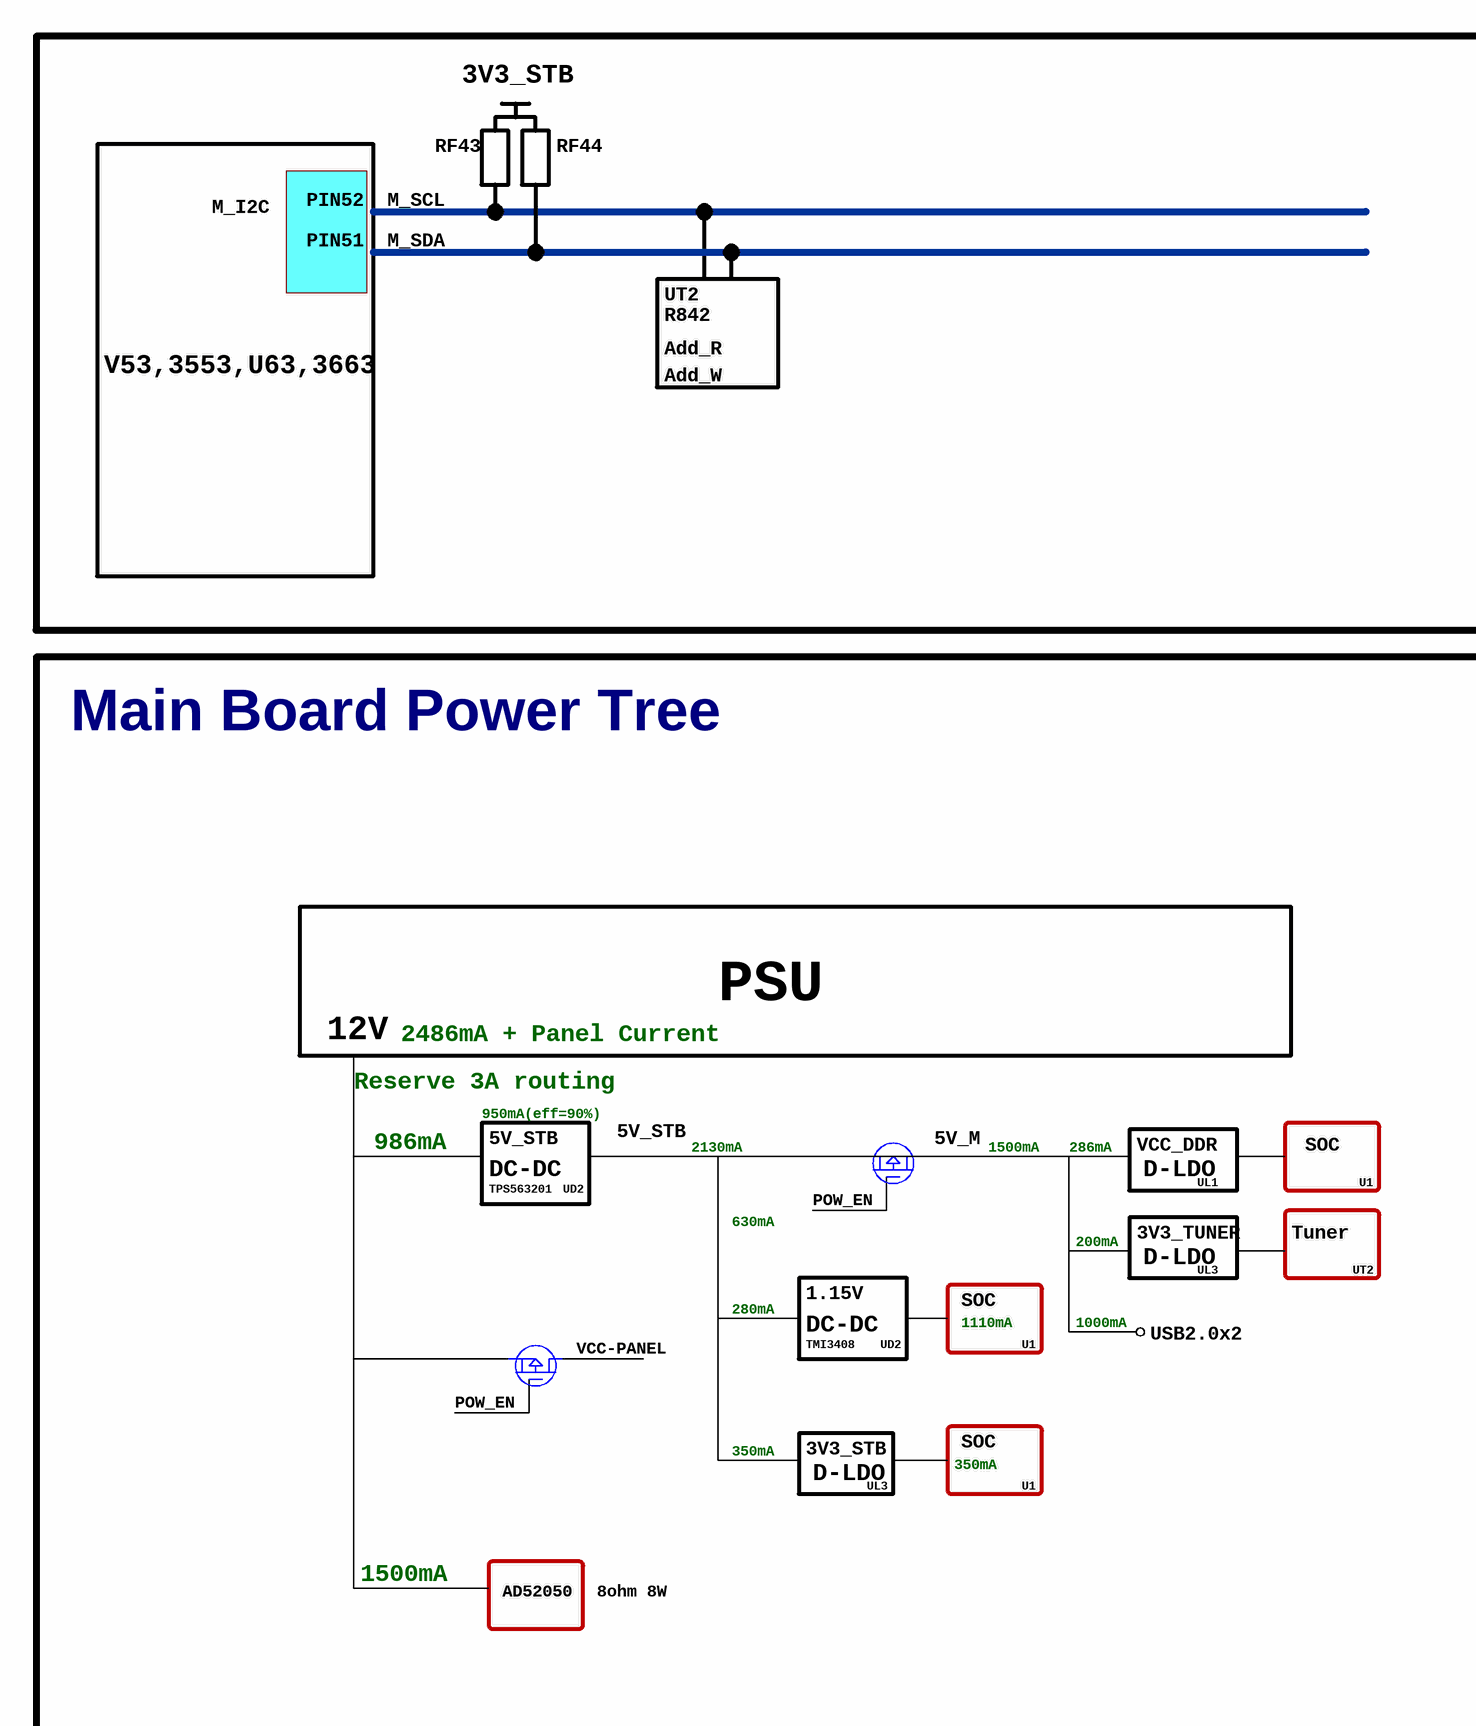
[diagram p0: MISC86372-17.SchDoc, left]
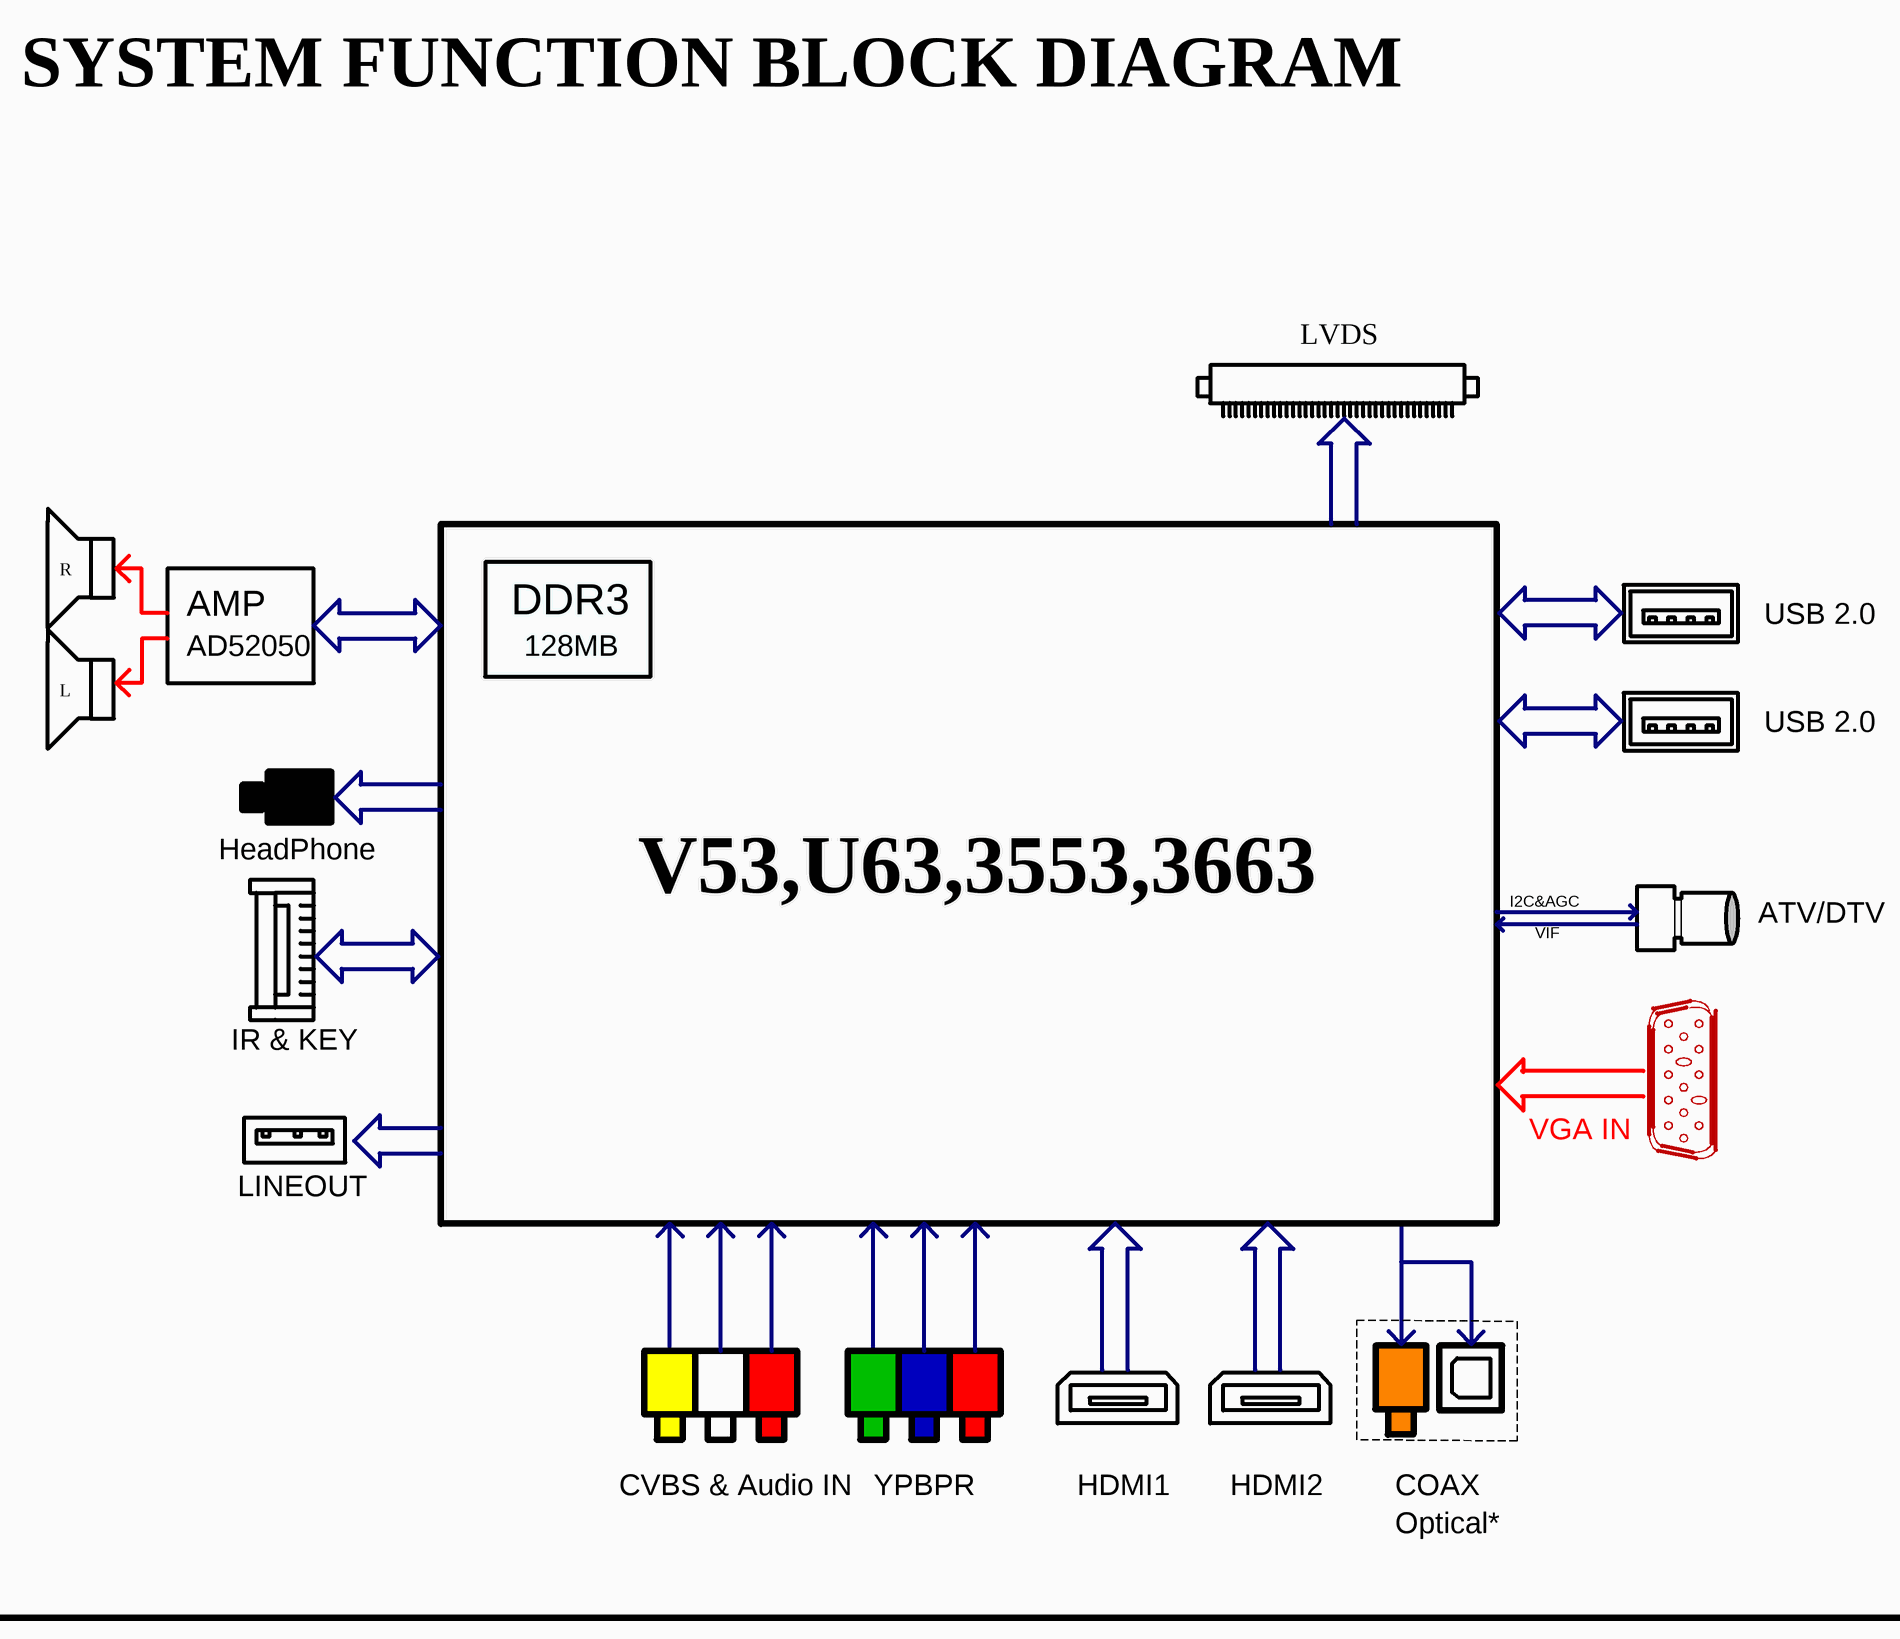
[diagram p1: MISC86372-17.SchDoc, right]
# Altium project MISC86372-32.PrjPCB (part 2 of 8)

## Sheet MISC86372-17.SchDoc
size 736 x 347 mm

### Notes on the sheet
- 3V3_STB
- RF43
- RF44
- SYSTEM FUNCTION BLOCK DIAGRAM
- M_I2C
- PIN52
- M_SCL
- PIN51
- M_SDA
- UT2
- V53,3553,U63,3663
- R842
- Add_R
- Add_W
- LVDS
- R
- Main Board Power Tree
- AMP
- AD52050
- DDR3
- 128MB
- USB 2.0
- L
- HeadPhone
- 12V
- 2486mA + Panel Current
- PSU
- V53,U63,3553,3663
- I2C&AGC
- ATV/DTV
- Reserve 3A routing
- VIF
- 986mA
- 950mA(eff=90%)
- DC-DC
- 5V_STB
- 2130mA
- 5V_M
- 1500mA
- 286mA
- VCC_DDR
- D-LDO
- UL1
- SOC
- U1
- IR & KEY
- TPS563201
- UD2
- 630mA
- POW_EN
- 200mA
- 3V3_TUNER
- Tuner
- 280mA
- 1.15V
- UL3
- VGA IN
- VCC-PANEL
- TMI3408
- 1110mA
- 1000mA
- USB2.0x2
- LINEOUT
- 350mA
- 8ohm 8W
- CVBS & Audio IN
- YPBPR
- HDMI1
- HDMI2
- COAX
- Optical*

## Sheet MISC86372-8.SchDoc
size 393 x 241 mm
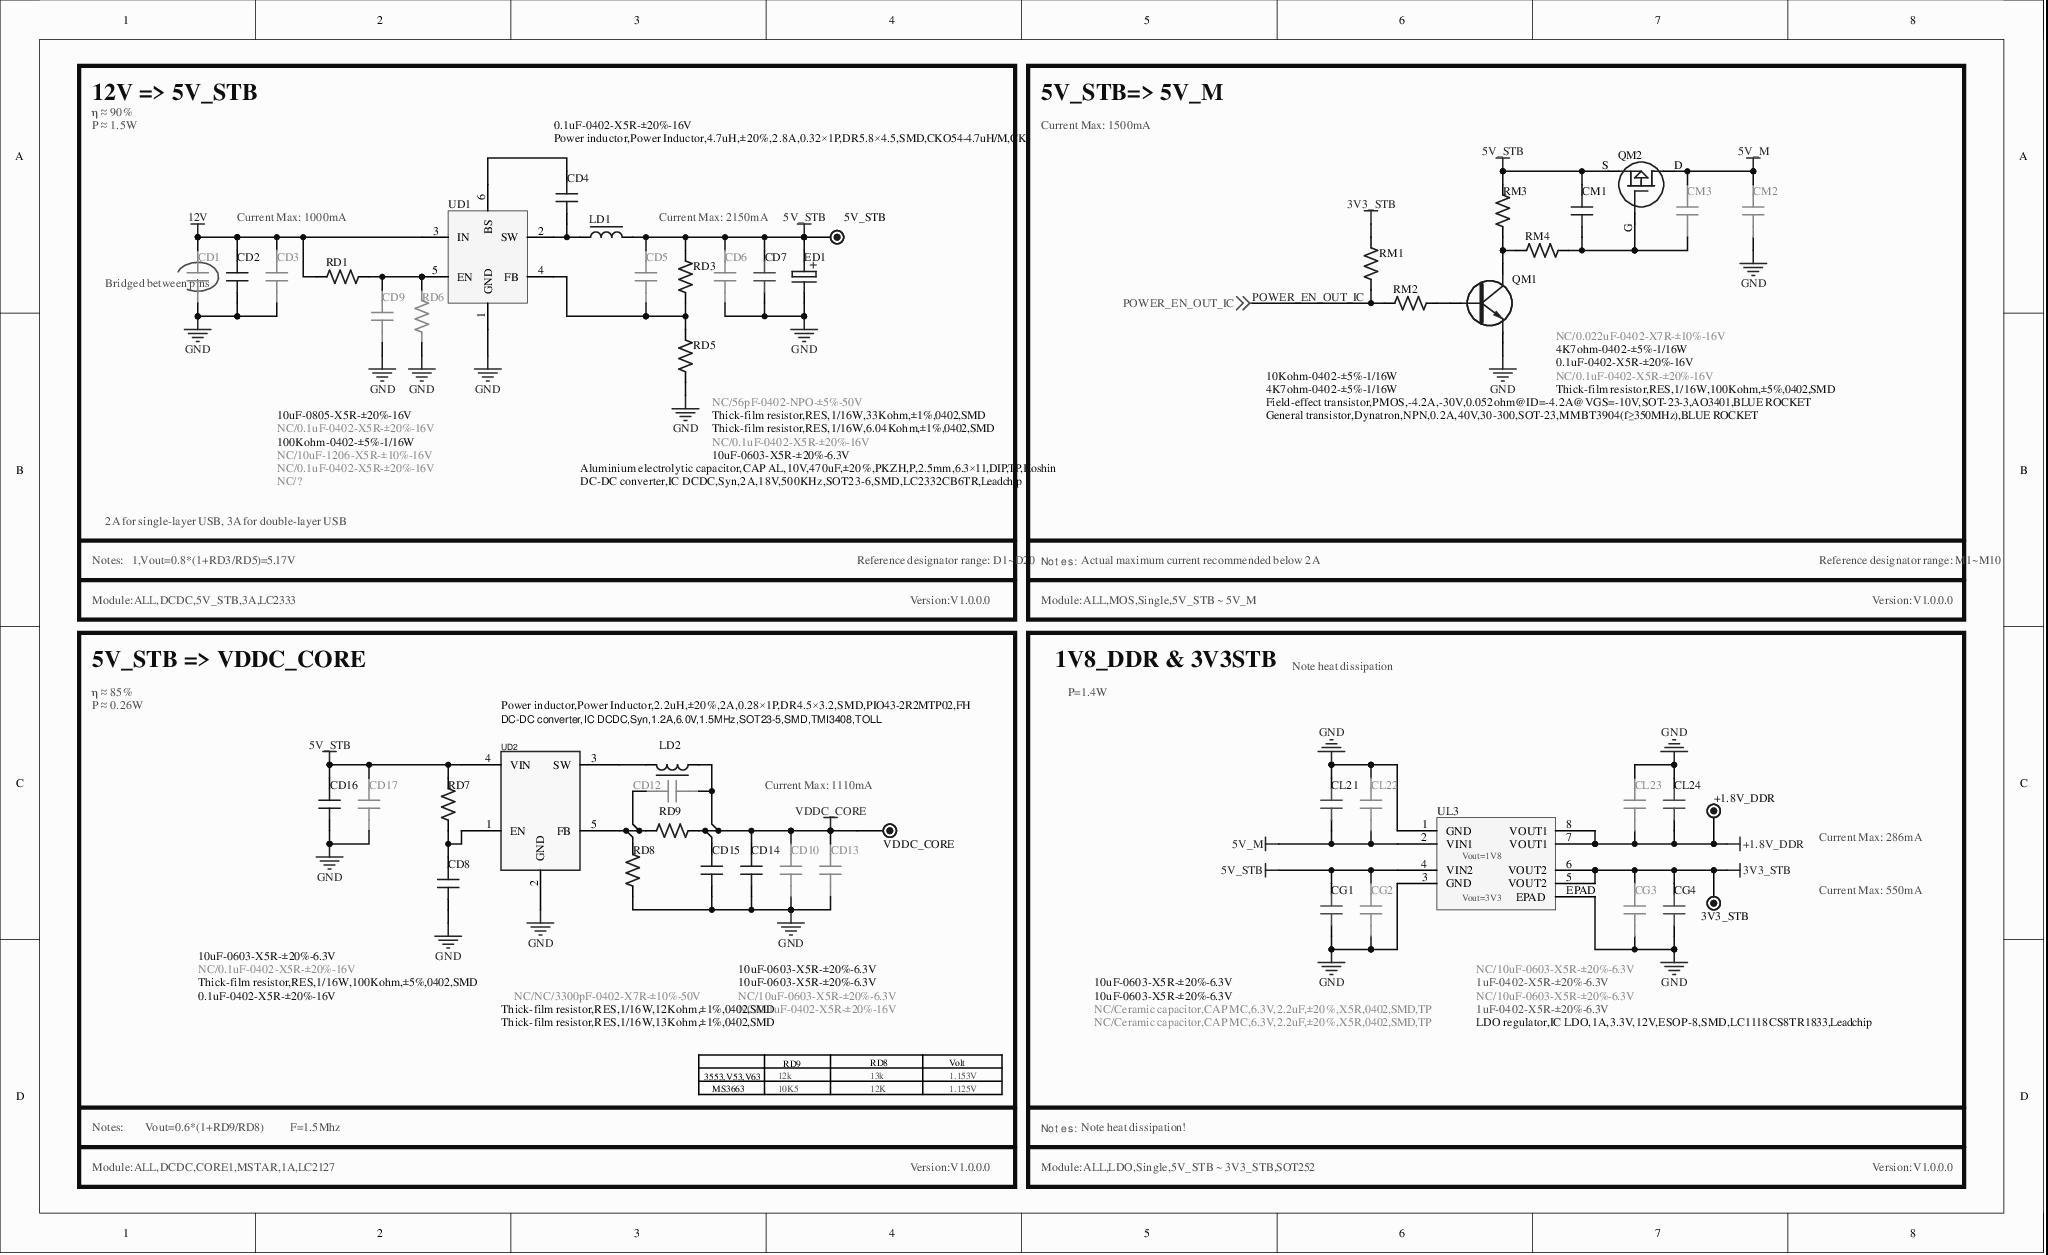
[diagram p2: MISC86372-8.SchDoc]

### Parts
3V3_STB  TEST  [TP]  (value not drawn)
5V_STB  TEST  [TP]  (value not drawn)
+1.8V_DDR  TEST  [TP]  (value not drawn)
CD1  NC/10uF-1206-X5R-±10%-16V  [C1206]
CD2  10uF-0805-X5R-±20%-16V  [C0805]
CD3  NC/0.1uF-0402-X5R-±20%-16V  [C0402]
CD4  0.1uF-0402-X5R-±20%-16V  [C0402]
CD5  NC/56pF-0402-NPO-±5%-50V  [C0402]
CD6  NC/0.1uF-0402-X5R-±20%-16V  [C0402]
CD7  10uF-0603-X5R-±20%-6.3V  [C0603]
CD8  0.1uF-0402-X5R-±20%-16V  [C0402]
CD9  NC/0.1uF-0402-X5R-±20%-16V  [C0402]
CD10  NC/10uF-0603-X5R-±20%-6.3V  [C0603]
CD12  NC/NC/3300pF-0402-X7R-±10%-50V  [C0402]
CD13  NC/0.1uF-0402-X5R-±20%-16V  [C0402]
CD14  10uF-0603-X5R-±20%-6.3V  [C0603]
CD15  10uF-0603-X5R-±20%-6.3V  [C0603]
CD16  10uF-0603-X5R-±20%-6.3V  [C0603]
CD17  NC/0.1uF-0402-X5R-±20%-16V  [C0402]
CG1  10uF-0603-X5R-±20%-6.3V  [C0603]
CG2  NC/Ceramic capacitor,CAP MC,6.3V,2.2uF,±20%,X5R,0402,SMD,TP  [C0402]
CG3  NC/10uF-0603-X5R-±20%-6.3V  [C0603]
CG4  1uF-0402-X5R-±20%-6.3V  [C0402]
CL21  10uF-0603-X5R-±20%-6.3V  [C0603]
CL22  NC/Ceramic capacitor,CAP MC,6.3V,2.2uF,±20%,X5R,0402,SMD,TP  [C0402]
CL23  NC/10uF-0603-X5R-±20%-6.3V  [C0603]
CL24  1uF-0402-X5R-±20%-6.3V  [C0402]
CM1  0.1uF-0402-X5R-±20%-16V  [C0402]
CM2  NC/0.1uF-0402-X5R-±20%-16V  [C0402]
CM3  NC/0.022uF-0402-X7R-±10%-16V  [C0402]
ED1  Aluminium electrolytic capacitor,CAP AL,10V,470uF,±20%,PKZH,P,2.5mm,6.3×11,DIP,TP,Koshin  [EC(6.3*11)-V-2.5]
LD1  Power inductor,Power Inductor,4.7uH,±20%,2.8A,0.32×1P,DR5.8×4.5,SMD,CKO54-4.7uH/M,CK  [L(5.8*4.5)-S]
LD2  Power inductor,Power Inductor,2.2uH,±20%,2A,0.28×1P,DR4.5×3.2,SMD,PIO43-2R2MTP02,FH  [L(4.5*3.5)-S]
QM1  General transistor,Dynatron,NPN,0.2A,40V,30-300,SOT-23,MMBT3904(f≥350MHz),BLUE ROCKET  [SOT-23]
QM2  Field-effect transistor,PMOS,-4.2A,-30V,0.052ohm@ID=-4.2A@VGS=-10V,SOT-23-3,AO3401,BLUE ROCKET  [SOT-23-1]
RD1  100Kohm-0402-±5%-1/16W  [R0402]
RD3  Thick-film resistor,RES,1/16W,33Kohm,±1%,0402,SMD  [R0402]
RD5  Thick-film resistor,RES,1/16W,6.04Kohm,±1%,0402,SMD  [R0402]
RD6  NC/?  [R0402]
RD7  Thick-film resistor,RES,1/16W,100Kohm,±5%,0402,SMD  [R0402]
RD8  Thick-film resistor,RES,1/16W,13Kohm,±1%,0402,SMD  [R0402]
RD9  Thick-film resistor,RES,1/16W,12Kohm,±1%,0402,SMD  [R0402]
RM1  10Kohm-0402-±5%-1/16W  [R0402]
RM2  4K7ohm-0402-±5%-1/16W  [R0402]
RM3  4K7ohm-0402-±5%-1/16W  [R0402]
RM4  Thick-film resistor,RES,1/16W,100Kohm,±5%,0402,SMD  [R0402]
UD1  DC-DC converter,IC DCDC,Syn,2A,18V,500KHz,SOT23-6,SMD,LC2332CB6TR,Leadchip  [SOT-23-6]
UD2  DC-DC converter,IC DCDC,Syn,1.2A,6.0V,1.5MHz,SOT23-5,SMD,TMI3408,TOLL  [SOT-23-5]
UL3  LDO regulator,IC LDO,1A,3.3V,12V,ESOP-8,SMD,LC1118CS8TR1833,Leadchip  [SOP8/1.27-3]
VDDC_CORE  TEST  [TP]  (value not drawn)

### Blocks framed on the sheet
12V => 5V_STB: 5V_STB CD1-CD7 CD9 ED1 LD1 RD1 RD3 RD5 RD6 UD1
5V_STB=> 5V_M: CM1-CM3 QM1 QM2 RM1-RM4
5V_STB => VDDC_CORE: CD8 CD10 CD12-CD17 LD2 RD7-RD9 UD2 VDDC_CORE
1V8_DDR & 3V3STB: 3V3_STB +1.8V_DDR CG1-CG4 CL21-CL24 UL3

### Nets
3V3_STB: 3V3_STB.1 CG3.2 CG4.1 RM1.2 UL3.5(VOUT2) UL3.6(VOUT2)
5V_M: CL21.1 CL22.1 CM2.2 CM3.1 QM2.D UL3.2(VIN1)
5V_STB: 5V_STB.1 CD5.2 CD6.2 CD7.2 CD16.2 CD17.2 CG1.2 CG2.2 CM1.2 ED1.1 LD1.2 QM2.S RD3.2 RD7.2 RM3.2 UD2.4(VIN) UL3.4(VIN2)
12V: CD1.2 CD2.1 CD3.2 RD1.1 UD1.3(IN)
+1.8V_DDR: +1.8V_DDR.1 CL23.1 CL24.2 UL3.7(VOUT1) UL3.8(VOUT1)
GND: CD1.1 CD2.2 CD3.1 CD6.1 CD7.1 CD8.1 CD9.1 CD10.1 CD13.1 CD14.1 CD15.1 CD16.1 CD17.1 CG1.1 CG2.1 CG3.1 CG4.2 CL21.2 CL22.2 CL23.2 CL24.1 CM2.1 ED1.2 QM1.E RD5.1 RD6.1 RD8.2 UD1.1(GND) UD2.2(GND) UL3.1(GND) UL3.3(GND) UL3.EPAD
VDDC_CORE: CD10.2 CD12.2 CD13.2 CD14.2 CD15.2 LD2.1 RD9.1 VDDC_CORE.1
POWER_EN_OUT_IC: RM1.1 RM2.1 ; off-sheet POWER_EN_OUT_IC
NetCD4_1: CD4.1 LD1.1 UD1.2(SW)
NetCD4_2: CD4.2 UD1.6(BS)
NetCD5_1: CD5.1 RD3.1 RD5.2 UD1.4(FB)
NetCD8_2: CD8.2 RD7.1 UD2.1(EN)
NetCD9_2: CD9.2 RD1.2 RD6.2 UD1.5(EN)
NetCD12_1: CD12.1 RD8.1 RD9.2 UD2.5(FB)
NetCM1_1: CM1.1 CM3.2 QM2.G RM4.2
NetLD2_2: LD2.2 UD2.3(SW)
NetQM1_B: QM1.B RM2.2
NetQM1_C: QM1.C RM3.1 RM4.1

### Notes on the sheet
- η ≈ 90%
- P ≈ 1.5W
- Current Max: 1500mA
- Current Max: 1000mA
- Current Max: 2150mA
- (near CD1) Bridged between pins
- 2A for single-layer USB, 3A for double-layer USB
- Module:ALL,DCDC,5V_STB,3A,LC2333
- Notes:
- 1,Vout=0.8*(1+RD3/RD5)=5.17V
- Reference designator range: D1~D20
- Version:V1.0.0.0
- Module:ALL,MOS,Single,5V_STB ~ 5V_M
- Actual maximum current recommended below 2A
- Reference designator range: M1~M10
- Note heat dissipation
- η ≈ 85%
- P ≈ 0.26W
- P=1.4W
- Current Max: 1110mA
- Current Max: 286mA
- Current Max: 550mA
- 3553,V53,V63
- 12k
- RD9
- RD8
- 13k
- Volt
- 1.153V
- Vout=0.6*(1+RD9/RD8)
- F=1.5Mhz
- MS3663
- 10K5
- 12K
- 1.125V
- Note heat dissipation!
- Module:ALL,DCDC,CORE1,MSTAR,1A,LC2127
- Module:ALL,LDO,Single,5V_STB ~ 3V3_STB,SOT252

### Library data of the parts
CD1 = 10uF-1206-X5R-±10%-16V-D
CD2 = 004.003.0000386-D: Ceramic capacitor,CAP MC,16V,10uF,±20%,X5R,0805,SMD,TP-D
CD3 CD4 CD6 CD8 CD9 CM1 CM2 = 004.003.0000403-D: Ceramic capacitor,CAP MC,16V,0.1uF,±20%,X5R,0402,SMD,TP-D
CD5 = 004.003.0000570-D: Ceramic capacitor,CAP MC,50V,56pF,±5%,NPO,0402,SMD,TP-D
CD7 CG1 CG3 CL21 CL23 = 004.003.0000383-D: Ceramic capacitor,CAP MC,6.3V,10uF,±20%,X5R,0603,SMD,TP-D
CD10 CD14-CD16 = 10uF-0603-X5R-±20%-6.3V-D
CD12 = 3300pF-0402-X7R-±10%-50V-D
CD13 CD17 = 0.1uF-0402-X5R-±20%-16V-D
CG2 CL22 = 004.003.0000100-D: Ceramic capacitor,CAP MC,6.3V,2.2uF,±20%,X5R,0402,SMD,TP-D
CG4 CL24 = 1uF-0402-X5R-±20%-6.3V-D
CM3 = 0.022uF-0402-X7R-±10%-16V-D
ED1 = 470uF-10V-±20%-6.3×11-105℃-黑底白字-编带-F=2.5-XF-DHAI: Electrolytic
LD1 = 004.004.0000017-D: Power inductor,Power Inductor,4.7uH,±20%,2.8A,0.35×1P,DR5.8×4.5,SMD,SCD54TL-4R7M,Soldier-D
LD2 = SLN43T-6R8M-D
QM1 = 004.006.0000007-D: General transistor,Dynatron,NPN,0.2A,40V,60-300,SOT-23,KMBT3904,KEXIN-D
QM2 = 004.007.0000286-D: Field-effect transistor,PMOS,-4.7A,-20V,70mohm@ID=-4.7A@VGS=-4.5V,SOT23-LC,LPB3443LT1G,LRC-D
RD1 RD7 RM4 = 004.002.0000579-D: Thick-film resistor,RES,1/16W,100Kohm,±5%,0402,SMD-D
RD3 = 004.002.0000104-D: Thick-film resistor,RES,1/16W,33Kohm,±1%,0402,SMD-D
RD5 = 004.002.0000717-D: Thick-film resistor,RES,1/16W,6.04Kohm,±1%,0402,SMD-D
RD6 = 004.002.0000806-D: Thick-film resistor,RES,1/16W,60.4Kohm,±1%,0402,SMD-D
RD8 = 004.002.0000593-D: Thick-film resistor,RES,1/16W,13Kohm,±1%,0402,SMD-D
RD9 = 004.002.0000588-D: Thick-film resistor,RES,1/16W,12Kohm,±1%,0402,SMD-D
RM1 RM2 = 004.002.0000577-D: Thick-film resistor,RES,1/16W,10Kohm,±5%,0402,SMD-D
RM3 = 004.002.0000689-D: Thick-film resistor,RES,1/16W,4.7Kohm,±5%,0402,SMD-D
UD1 = 004.010.0000700-D: DC-DC converter,IC DCDC,Syn,2A,18V,500KHz,SOT23-6,SMD,LC2332CB6TR,Leadchip-D
UD2 = DC-DC芯片,IC DCDC,Syn,1.2A,7.0V,1.5MHz,SOT23-5,SMD,LC2127CB5TR,Leadchip-D
UL3 = 004.010.0000256-D: LDO regulator,IC LDO,1A,3.3V,12V,ESOP-8,SMD,LC1118CS8TR1833,Leadchip-D